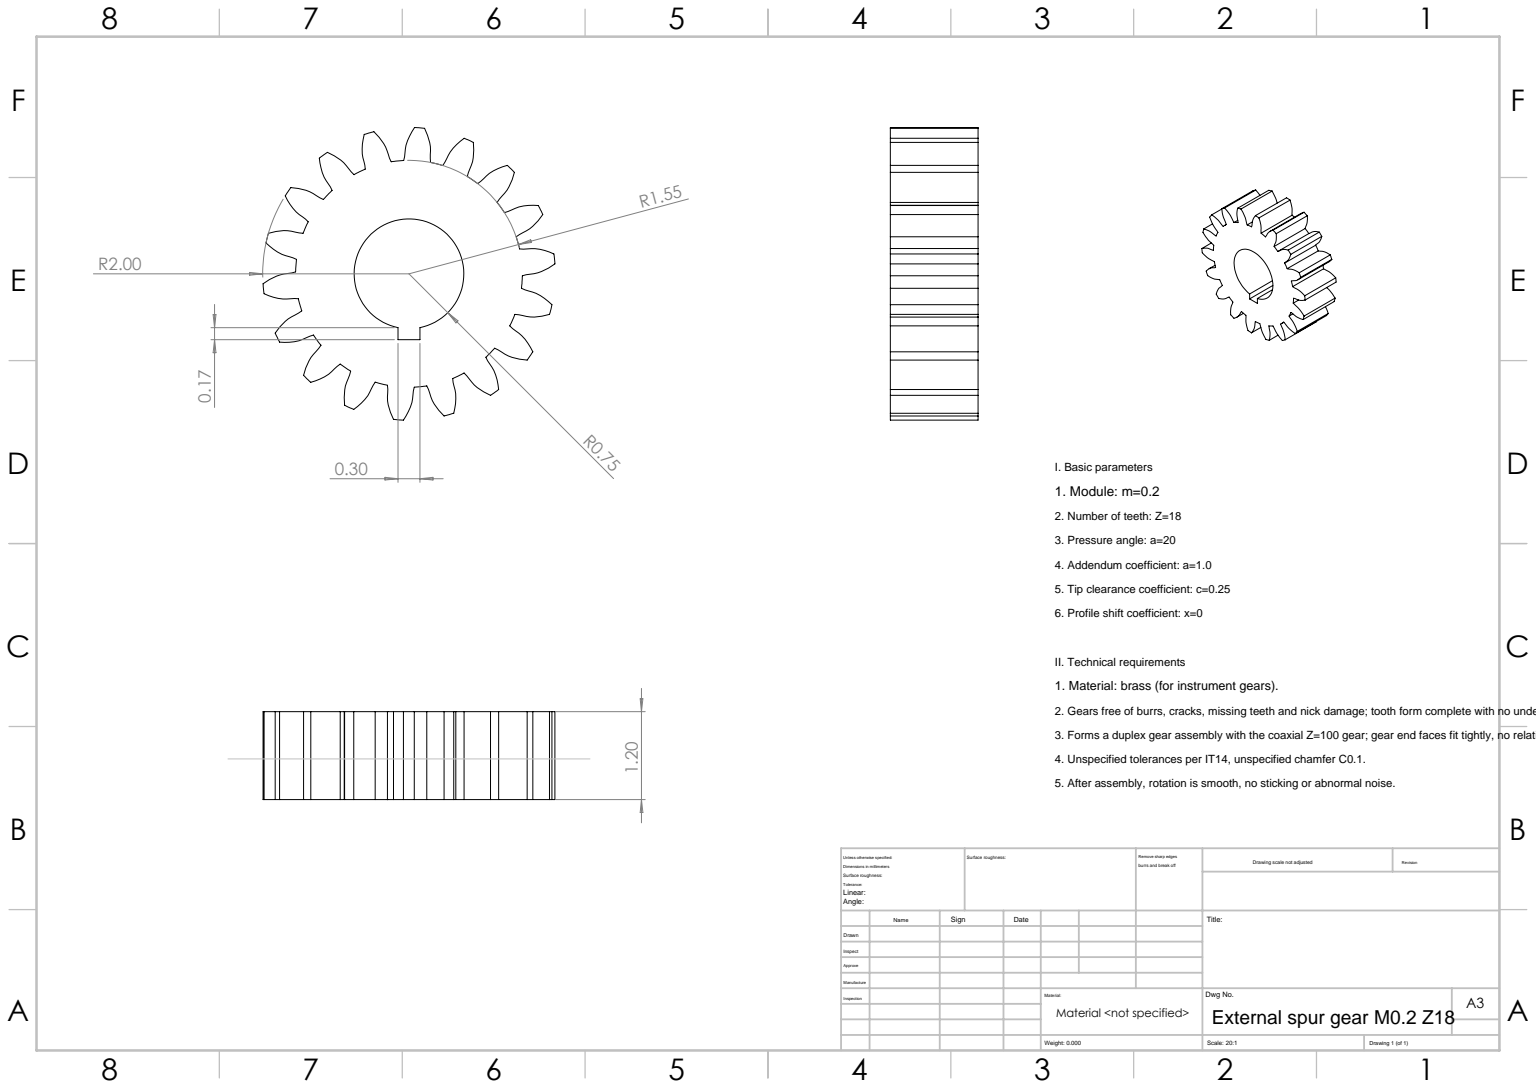
SolidWorks part; units mm, degrees
ref_plane "Front Plane" through (0, 0, 0) normal (0, 0, 1) x (1, 0, 0)
ref_plane "Top Plane" through (0, 0, 0) normal (0, 1, 0) x (1, 0, 0)
ref_plane "Right Plane" through (0, 0, 0) normal (1, 0, 0) x (0, 0, -1)
sketch "Sketch1" plane through (0, 0, 0) normal (0, 0, 1) x (1, 0, 0)
  circle A0 centre (0, 0) radius 1.55
  circle A1 centre (0, 0) radius 0.75
extrude "Boss-Extrude1" add sketch "Sketch1" along normal blind 1.2
sketch "Sketch2" plane through (0, 0, 0) normal (0, 0, 1) x (1, 0, 0)
  arc A0 (1.9815, 0.2717) -> (1.9954, 0.1361) centre (0, 0) cw
  arc A1 (1.5123, 0.34) -> (1.5498, -0.026) centre (0, 0) cw
  spline S0 degree 3 poles (1.9954, 0.1361) (1.9573, 0.1084) (1.8984, 0.0707) (1.8157, 0.0321) (1.7091, -0.0072) (1.6148, -0.0023) (1.5498, -0.026) knots 0 0 0 0 0.294269 0.434361 0.569741 1 1 1 1
  spline S1 degree 3 poles (1.9815, 0.2717) (1.9386, 0.2911) (1.8733, 0.316) (1.7844, 0.337) (1.6721, 0.3538) (1.5807, 0.33) (1.5123, 0.34) knots 0 0 0 0 0.294269 0.434361 0.569741 1 1 1 1
extrude "Boss-Extrude2" add sketch "Sketch2" along normal blind 1.2
pattern_circular "CirPattern1" count 18 over 360 about axis through (0, 0, 1.2) along (0, 0, -1) of "Boss-Extrude2"
sketch "Sketch3" plane through (0, 0, 1.2) normal (0, 0, 1) x (1, 0, 0)
  line L1 (0.15, -0.9) -> (-0.15, -0.9)
  line L2 (0.15, -0.9) -> (0.15, -0.6)
  line L3 (0.15, -0.6) -> (-0.15, -0.6)
  line L4 (-0.15, -0.9) -> (-0.15, -0.6)
  line L5 (0, -0.6) -> (0, -0.9) construction
  line L6 (0.15, -0.75) -> (-0.15, -0.75) construction
  circle A0 centre (0, 0) radius 0.75 construction
  point P0 (0, -0.75)
  dimension "D1" = 0.3
  dimension "D2" = 0.3
extrude "Cut-Extrude1" cut sketch "Sketch3" against normal blind 10
